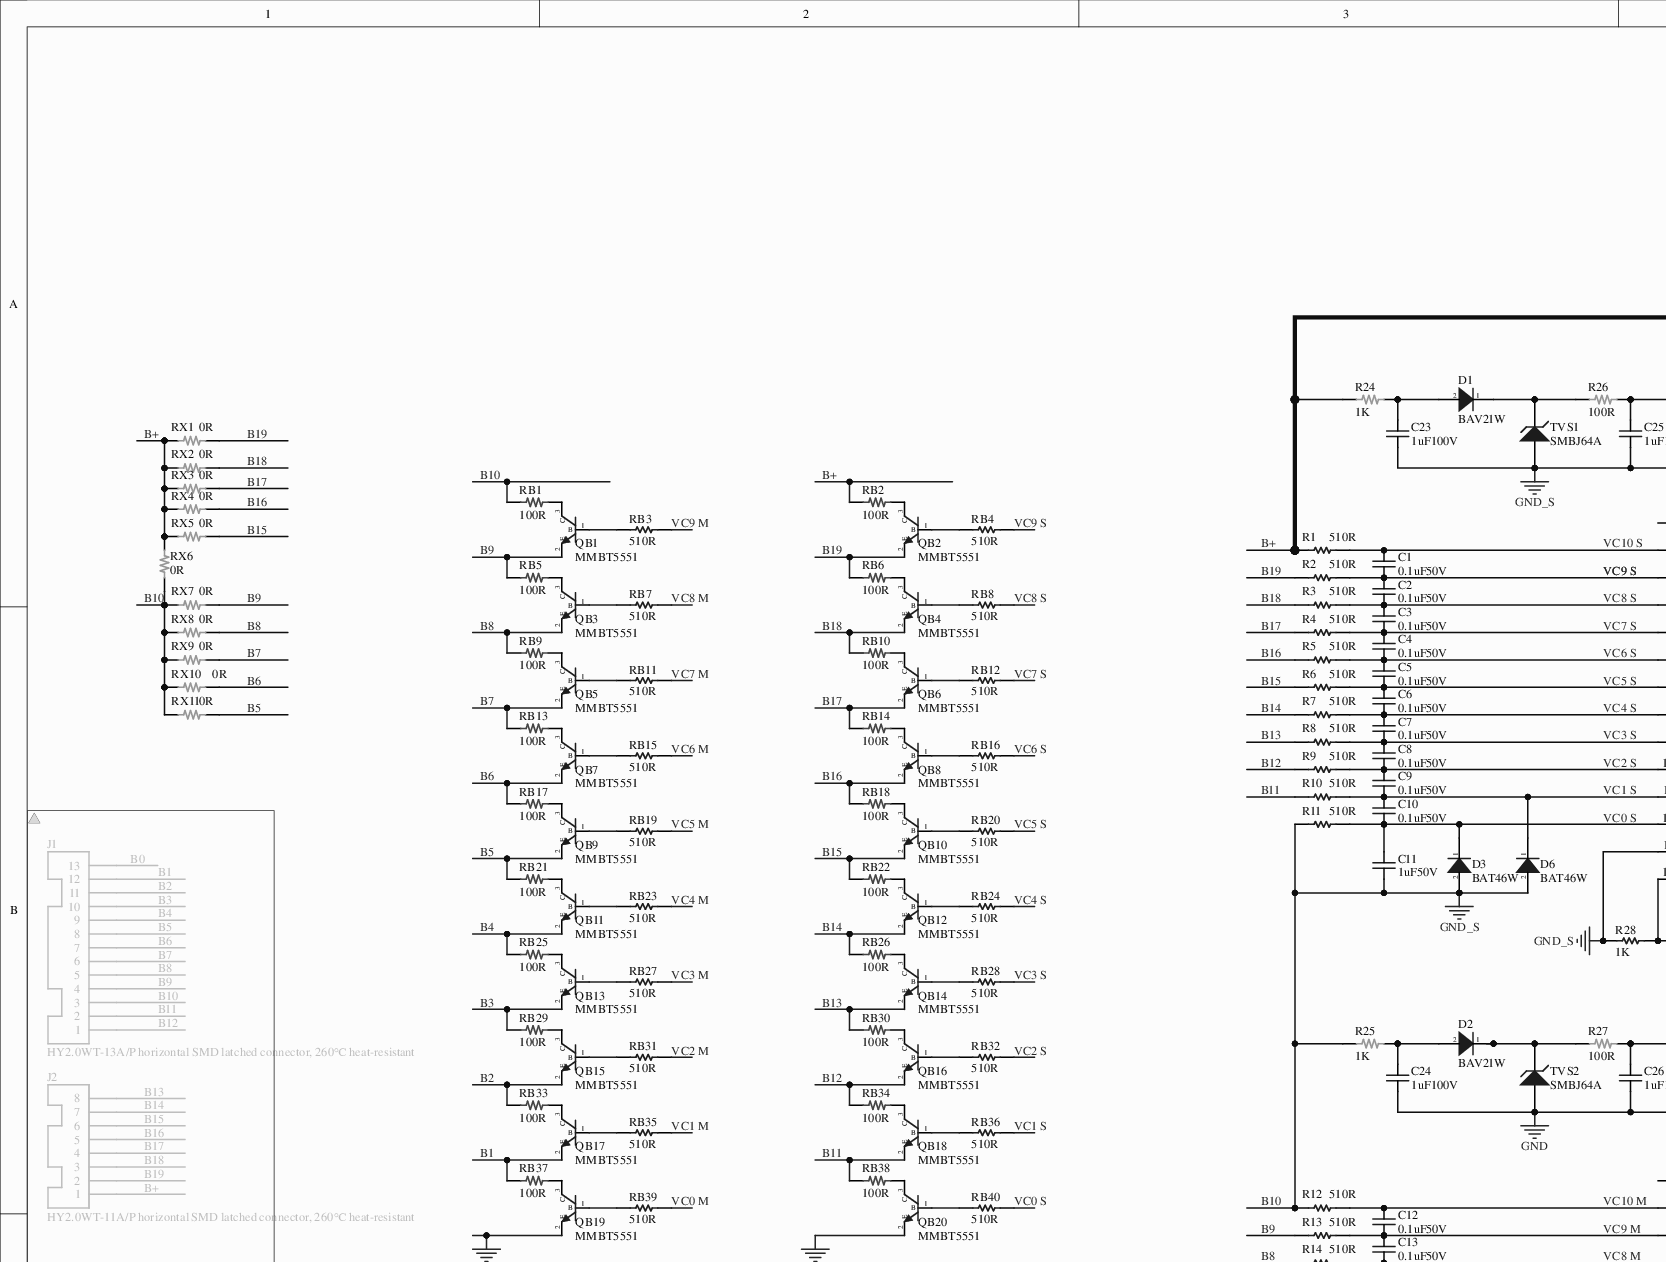
[diagram p0: MISC82749.SchDoc, top left]
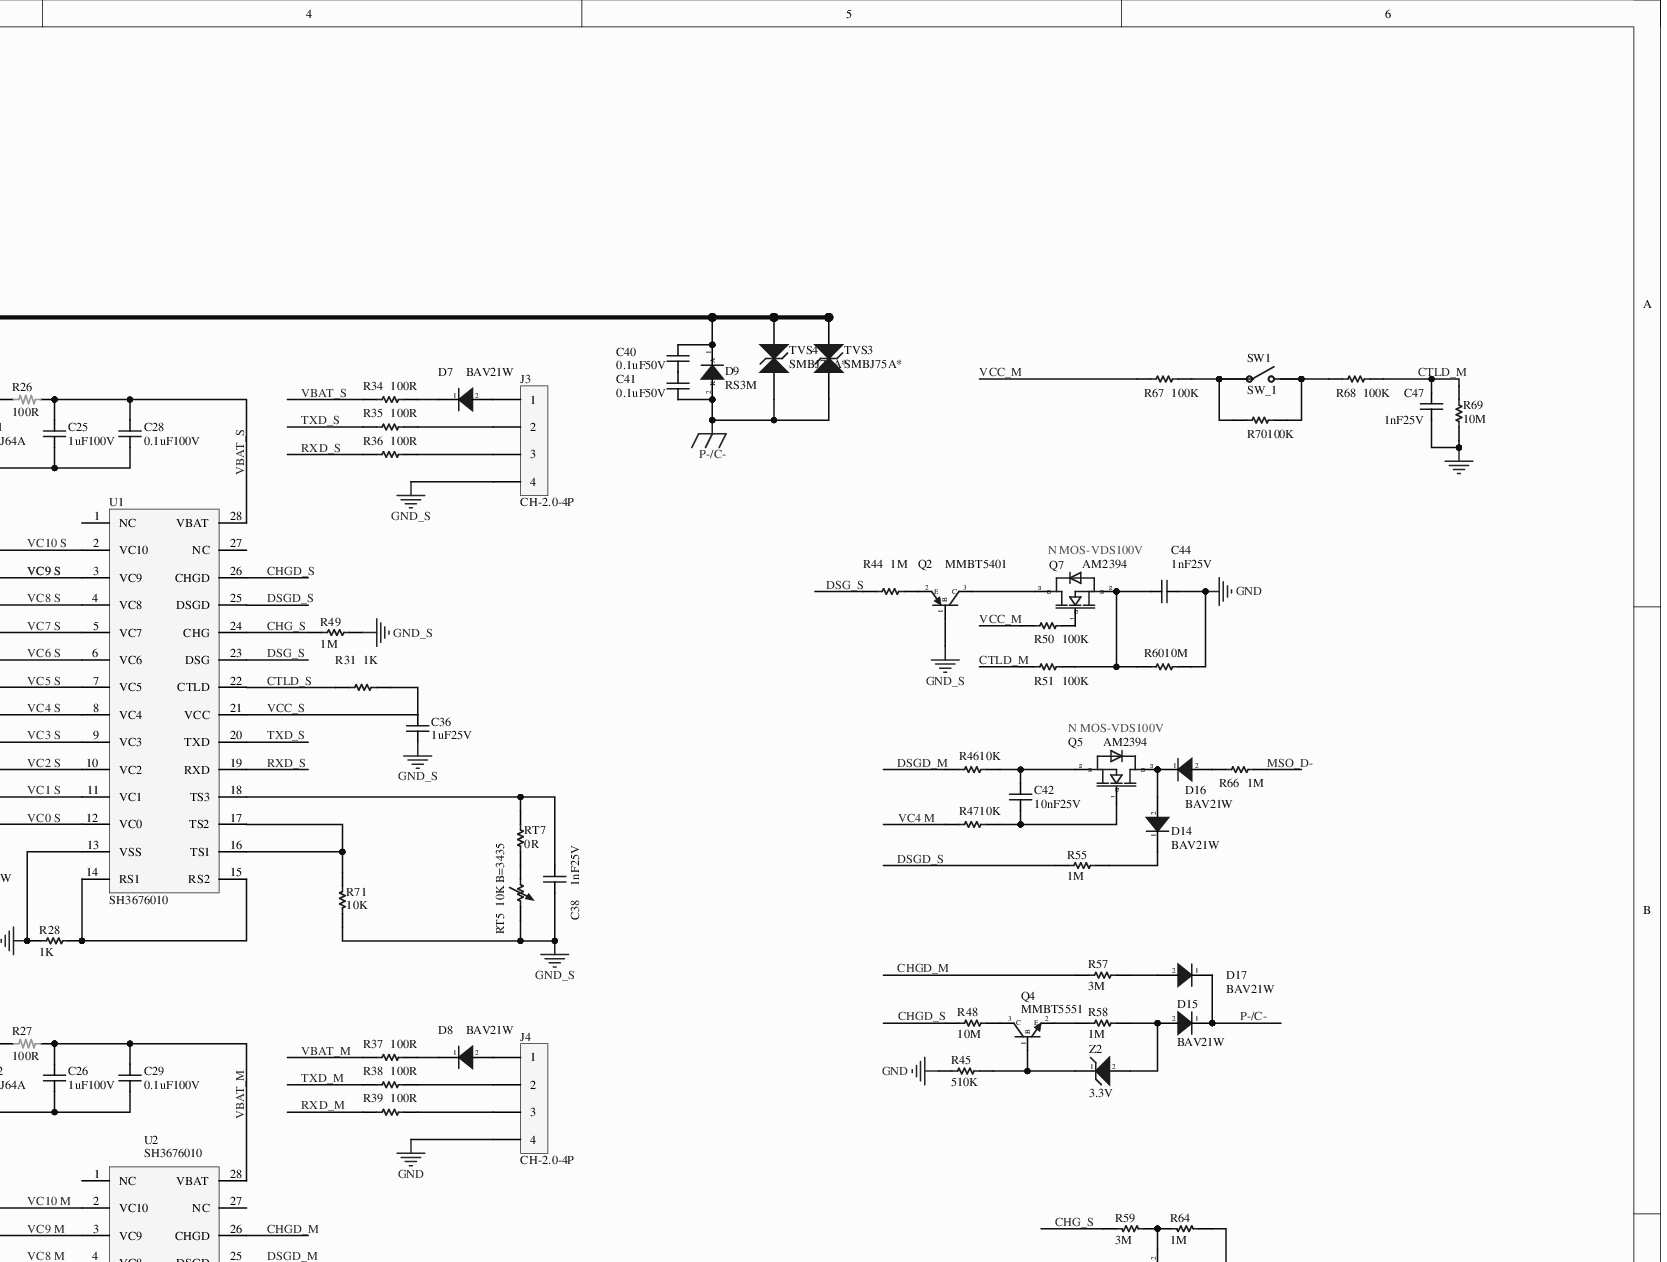
[diagram p1: MISC82749.SchDoc, top right]
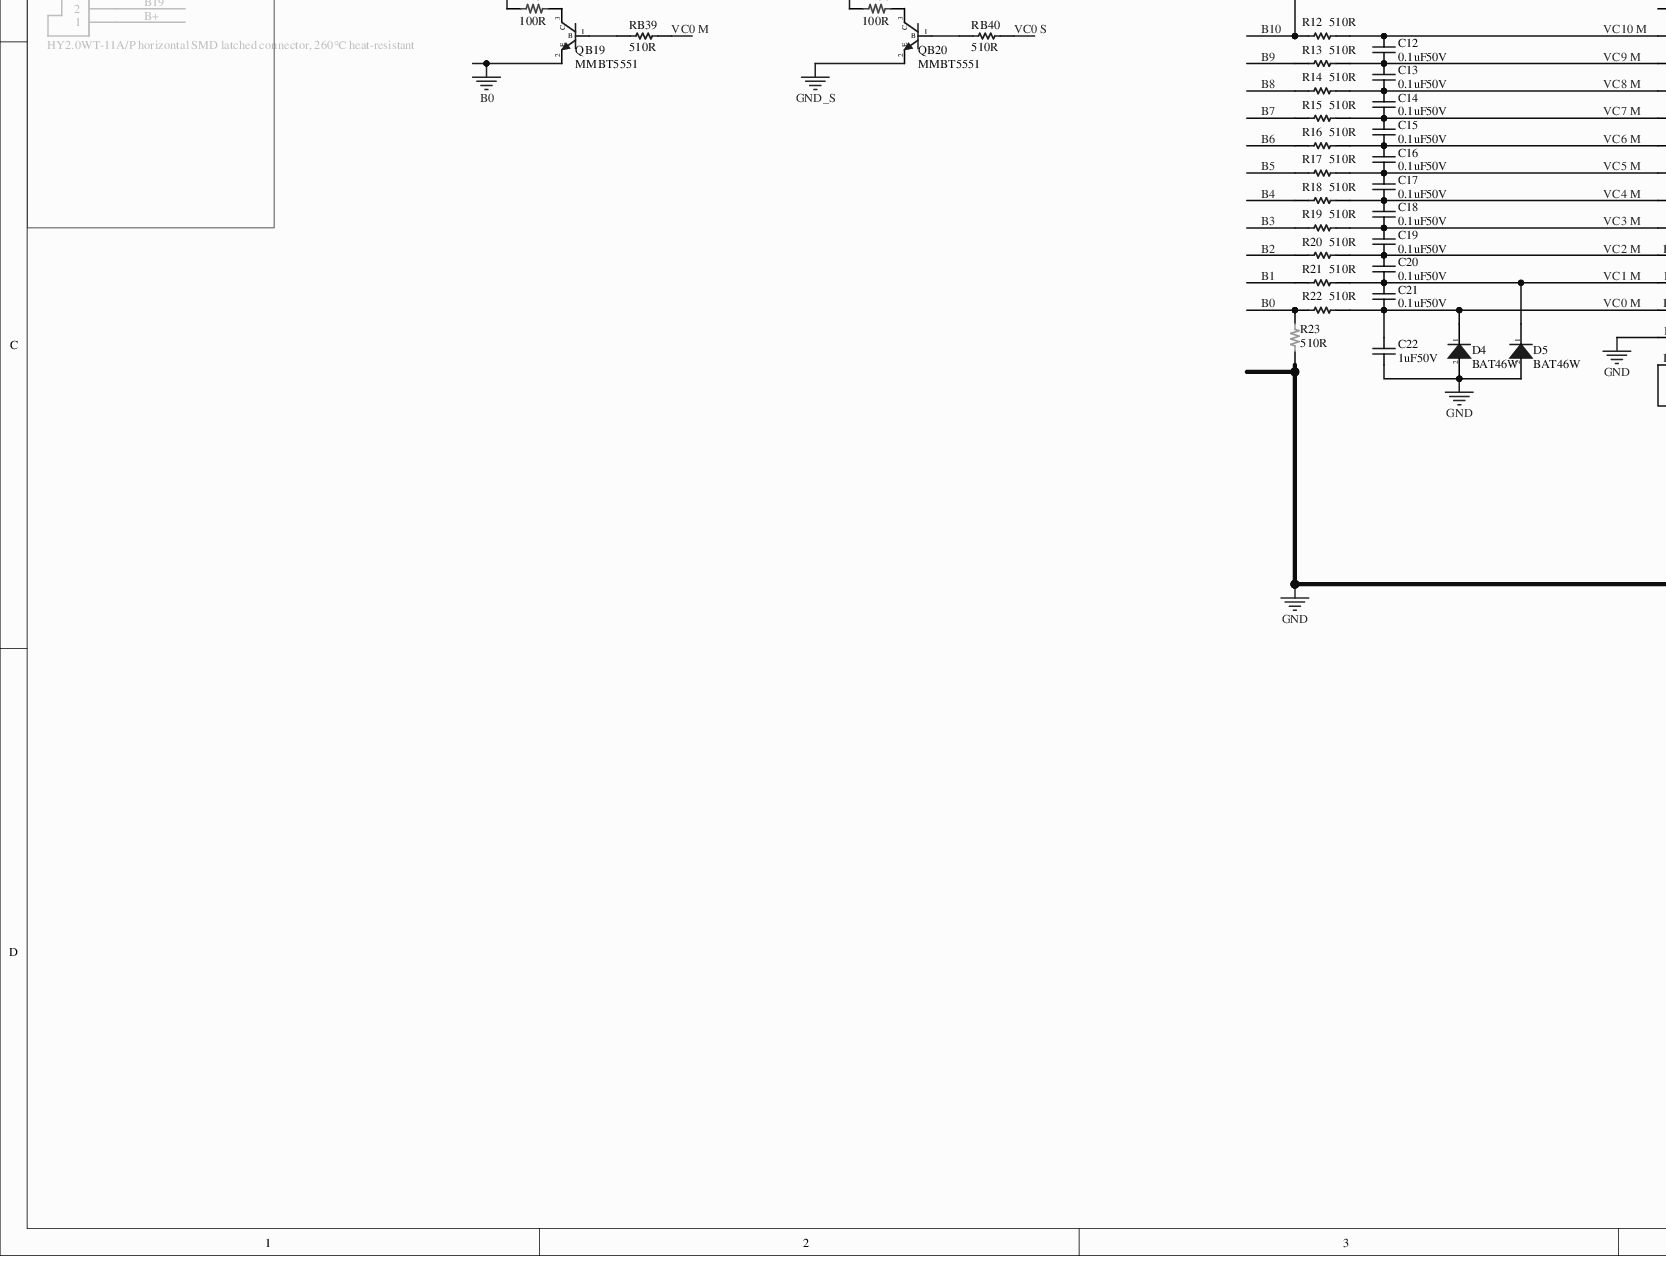
[diagram p2: MISC82749.SchDoc, bottom left]
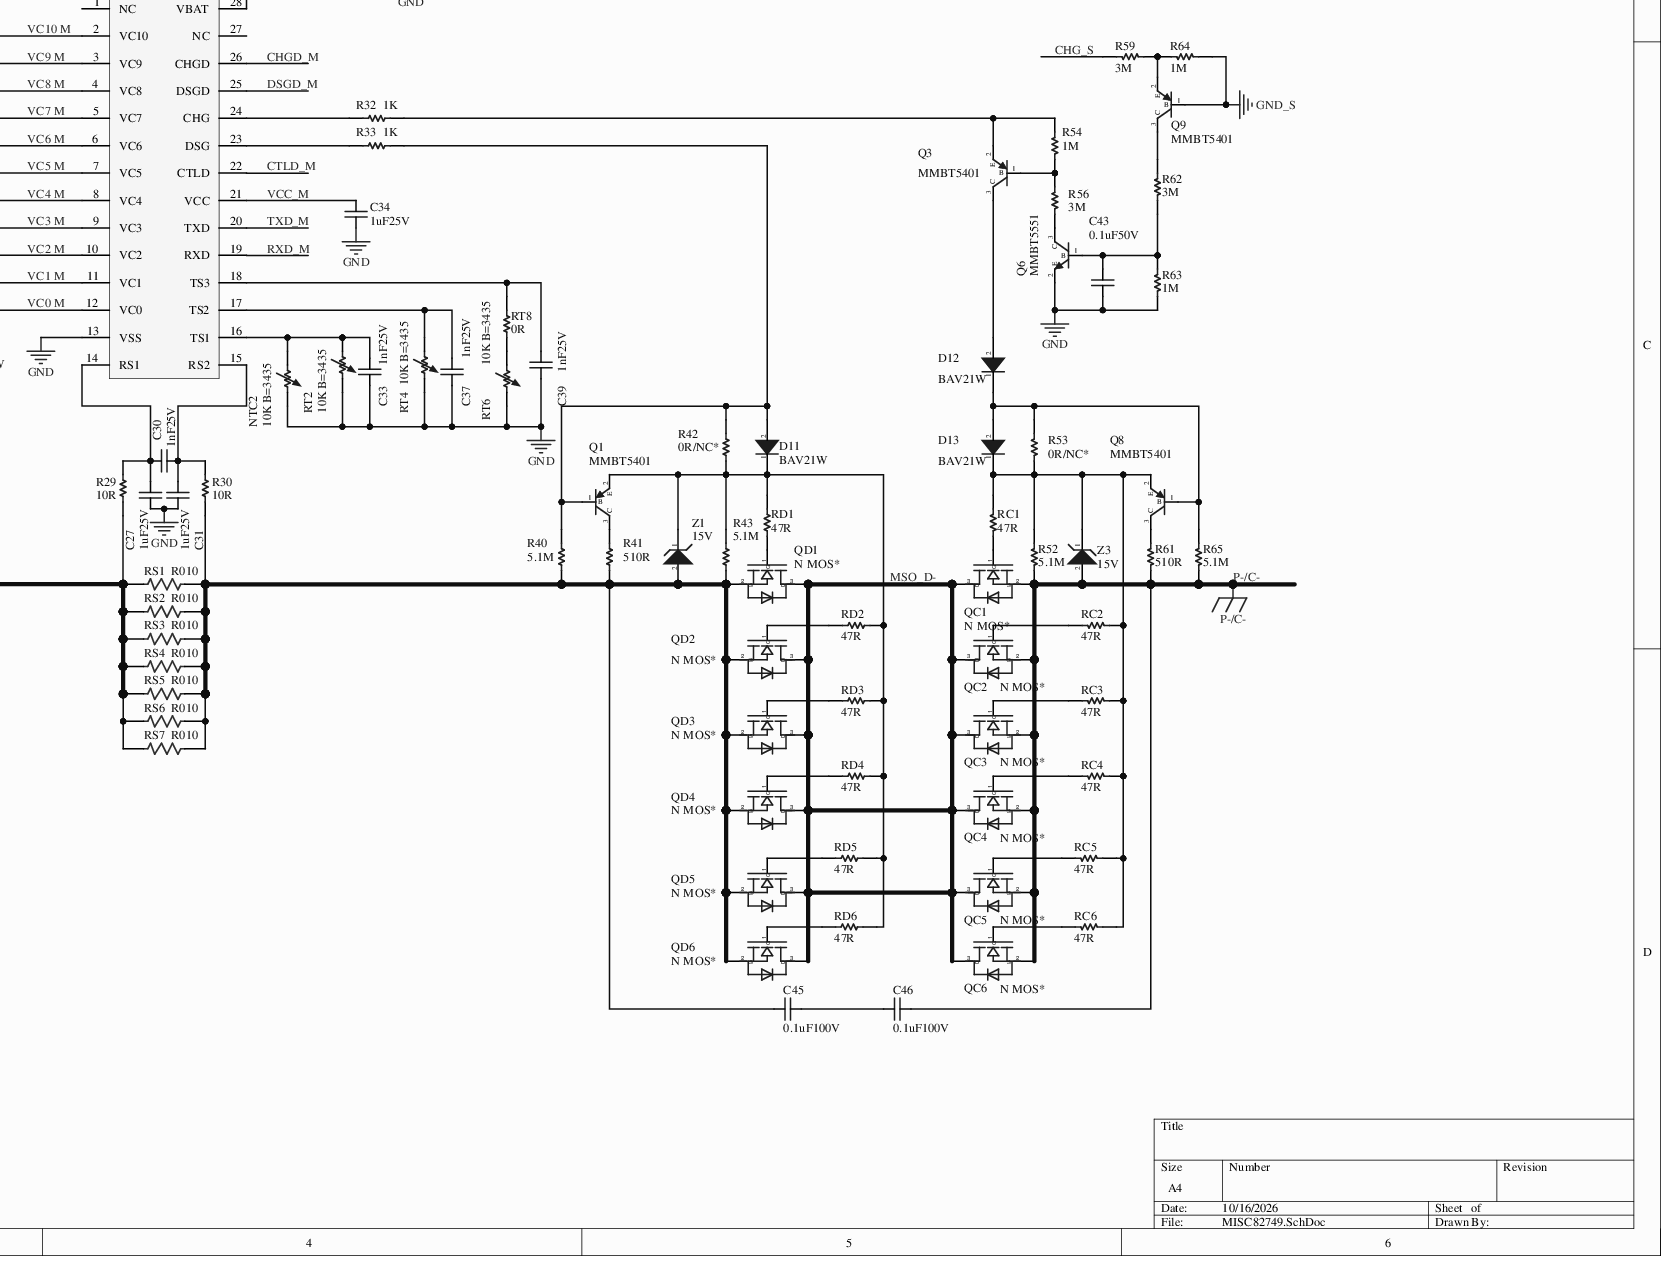
[diagram p3: MISC82749.SchDoc, bottom right]
# Altium project MISC82749.PrjPcb
1 sheet, 264 parts. Net scope: global (net labels, ports and power ports of the same name join across sheets).
Board file: MISC82749.PcbDoc

## Sheet MISC82749.SchDoc
size 599 x 449 mm; SheetNumber: 1; SheetTotal: 1

### Parts
C1  0.1uF50V  [C0603A]
C2  0.1uF50V  [C0603A]
C3  0.1uF50V  [C0603A]
C4  0.1uF50V  [C0603A]
C5  0.1uF50V  [C0603A]
C6  0.1uF50V  [C0603A]
C7  0.1uF50V  [C0603A]
C8  0.1uF50V  [C0603A]
C9  0.1uF50V  [C0603A]
C10  0.1uF50V  [C0603A]
C11  1uF50V  [C0603A]
C12  0.1uF50V  [C0603A]
C13  0.1uF50V  [C0603A]
C14  0.1uF50V  [C0603A]
C15  0.1uF50V  [C0603A]
C16  0.1uF50V  [C0603A]
C17  0.1uF50V  [C0603A]
C18  0.1uF50V  [C0603A]
C19  0.1uF50V  [C0603A]
C20  0.1uF50V  [C0603A]
C21  0.1uF50V  [C0603A]
C22  1uF50V  [C0603A]
C23  1uF100V  [C0805L]
C24  1uF100V  [C0805L]
C25  1uF100V  [C0805L]
C26  1uF100V  [C0805L]
C27  1uF25V  [C0603A]
C28  0.1uF100V  [C0805L]
C29  0.1uF100V  [C0805L]
C30  1nF25V  [C0603A]
C31  1uF25V  [C0603A]
C33  1nF25V  [C0603A]
C34  1uF25V  [C0603A]
C36  1uF25V  [C0603A]
C37  1nF25V  [C0603A]
C38  1nF25V  [C0603A]
C39  1nF25V  [C0603A]
C40  0.1uF50V  [C0603A]
C41  0.1uF50V  [C0603A]
C42  10nF25V  [C0603A]
C43  0.1uF50V  [C0603A]
C44  1nF25V  [C0603A]
C45  0.1uF100V  [C0603A]
C46  0.1uF100V  [C0603A]
C47  1nF25V  [C0603A]
D1  BAV21W  [SOD323A]
D2  BAV21W  [SOD323A]
D3  BAT46W  [SOD123]
D4  BAT46W  [SOD123]
D5  BAT46W  [SOD123]
D6  BAT46W  [SOD123]
D7  BAV21W  [SOD323A]
D8  BAV21W  [SOD323A]
D9  RS3M  [SMB A]
D11  BAV21W  [SOD323A]
D12  BAV21W  [SOD323A]
D13  BAV21W  [SOD323A]
D14  BAV21W  [SOD323A]
D15  BAV21W  [SOD323A]
D16  BAV21W  [SOD323A]
D17  BAV21W  [SOD323A]
J1  HY2.0WT-13A/P horizontal SMD latched connector, 260℃ heat-resistant  [2.0-13PIN直针带扣连接器]  (masked out: inside a compile mask, not in the netlist)
J2  HY2.0WT-11A/P horizontal SMD latched connector, 260℃ heat-resistant  [2.0-8PIN直针带扣连接器]  (masked out: inside a compile mask, not in the netlist)
J3  CH-2.0-4P  [Test2.0-4P]
J4  CH-2.0-4P  [Test2.0-4P]
NTC2  10K B=3435  [RT2.3X1.2-2]
Q1  MMBT5401  [SOT23-3]
Q2  MMBT5401  [SOT23-3]
Q3  MMBT5401  [SOT23-3]
Q4  MMBT5551  [SOT23-3]
Q5  AM2394  [SOT23-3L]
Q6  MMBT5551  [SOT23-3]
Q7  AM2394  [SOT23-3L]
Q8  MMBT5401  [SOT23-3]
Q9  MMBT5401  [SOT23-3]
QB1  MMBT5551  [SOT23-3]
QB2  MMBT5551  [SOT23-3]
QB3  MMBT5551  [SOT23-3]
QB4  MMBT5551  [SOT23-3]
QB5  MMBT5551  [SOT23-3]
QB6  MMBT5551  [SOT23-3]
QB7  MMBT5551  [SOT23-3]
QB8  MMBT5551  [SOT23-3]
QB9  MMBT5551  [SOT23-3]
QB10  MMBT5551  [SOT23-3]
QB11  MMBT5551  [SOT23-3]
QB12  MMBT5551  [SOT23-3]
QB13  MMBT5551  [SOT23-3]
QB14  MMBT5551  [SOT23-3]
QB15  MMBT5551  [SOT23-3]
QB16  MMBT5551  [SOT23-3]
QB17  MMBT5551  [SOT23-3]
QB18  MMBT5551  [SOT23-3]
QB19  MMBT5551  [SOT23-3]
QB20  MMBT5551  [SOT23-3]
QC1  N MOS*  [TOLL_123]
QC2  N MOS*  [TOLL_123]
QC3  N MOS*  [TOLL_123]
QC4  N MOS*  [TOLL_123]
QC5  N MOS*  [TOLL_123]
QC6  N MOS*  [TOLL_123]
QD1  N MOS*  [TOLL_123]
QD2  N MOS*  [TOLL_123]
QD3  N MOS*  [TOLL_123]
QD4  N MOS*  [TOLL_123]
QD5  N MOS*  [TOLL_123]
QD6  N MOS*  [TOLL_123]
R1  510R  [R0603A]
R2  510R  [R0603A]
R3  510R  [R0603A]
R4  510R  [R0603A]
R5  510R  [R0603A]
R6  510R  [R0603A]
R7  510R  [R0603A]
R8  510R  [R0603A]
R9  510R  [R0603A]
R10  510R  [R0603A]
R11  510R  [R0603A]
R12  510R  [R0603A]
R13  510R  [R0603A]
R14  510R  [R0603A]
R15  510R  [R0603A]
R16  510R  [R0603A]
R17  510R  [R0603A]
R18  510R  [R0603A]
R19  510R  [R0603A]
R20  510R  [R0603A]
R21  510R  [R0603A]
R22  510R  [R0603A]
R23  510R  [R0805L]
R24  1K  [R0805L]
R25  1K  [R0805L]
R26  100R  [R0805L]
R27  100R  [R0805L]
R28  1K  [R0603A]
R29  10R  [R0603A]
R30  10R  [R0603A]
R31  1K  [R0603A]
R32  1K  [R0603A]
R33  1K  [R0603A]
R34  100R  [R0603A]
R35  100R  [R0603A]
R36  100R  [R0603A]
R37  100R  [R0603A]
R38  100R  [R0603A]
R39  100R  [R0603A]
R40  5.1M  [R0603A]
R41  510R  [R0603A]
R42  0R/NC*  [R0603A]
R43  5.1M  [R0603A]
R44  1M  [R0603A]
R45  510K  [R0603A]
R46  10K  [R0603A]
R47  10K  [R0603A]
R48  10M  [R0603A]
R49  1M  [R0603A]
R50  100K  [R0603A]
R51  100K  [R0603A]
R52  5.1M  [R0603A]
R53  0R/NC*  [R0603A]
R54  1M  [R0603A]
R55  1M  [R0603A]
R56  3M  [R0603A]
R57  3M  [R0603A]
R58  1M  [R0603A]
R59  3M  [R0603A]
R60  10M  [R0603A]
R61  510R  [R0603A]
R62  3M  [R0603A]
R63  1M  [R0603A]
R64  1M  [R0603A]
R65  5.1M  [R0603A]
R66  1M  [R0603A]
R67  100K  [R0603A]
R68  100K  [R0603A]
R69  10M  [R0603A]
R70  100K  [R0603A]
R71  10K  [R0603A]
RB1  100R  [R1206A]
RB2  100R  [R1206A]
RB3  510R  [R0603A]
RB4  510R  [R0603A]
RB5  100R  [R1206A]
RB6  100R  [R1206A]
RB7  510R  [R0603A]
RB8  510R  [R0603A]
RB9  100R  [R1206A]
RB10  100R  [R1206A]
RB11  510R  [R0603A]
RB12  510R  [R0603A]
RB13  100R  [R1206A]
RB14  100R  [R1206A]
RB15  510R  [R0603A]
RB16  510R  [R0603A]
RB17  100R  [R1206A]
RB18  100R  [R1206A]
RB19  510R  [R0603A]
RB20  510R  [R0603A]
RB21  100R  [R1206A]
RB22  100R  [R1206A]
RB23  510R  [R0603A]
RB24  510R  [R0603A]
RB25  100R  [R1206A]
RB26  100R  [R1206A]
RB27  510R  [R0603A]
RB28  510R  [R0603A]
RB29  100R  [R1206A]
RB30  100R  [R1206A]
RB31  510R  [R0603A]
RB32  510R  [R0603A]
RB33  100R  [R1206A]
RB34  100R  [R1206A]
RB35  510R  [R0603A]
RB36  510R  [R0603A]
RB37  100R  [R1206A]
RB38  100R  [R1206A]
RB39  510R  [R0603A]
RB40  510R  [R0603A]
RC1  47R  [R0603A]
RC2  47R  [R0603A]
RC3  47R  [R0603A]
RC4  47R  [R0603A]
RC5  47R  [R0603A]
RC6  47R  [R0603A]
RD1  47R  [R0603A]
RD2  47R  [R0603A]
RD3  47R  [R0603A]
RD4  47R  [R0603A]
RD5  47R  [R0603A]
RD6  47R  [R0603A]
RS1  R010  [R2512L]
RS2  R010  [R2512L]
RS3  R010  [R2512L]
RS4  R010  [R2512L]
RS5  R010  [R2512L]
RS6  R010  [R2512L]
RS7  R010  [R2512L]
RT2  10K B=3435  [R0603A]
RT4  10K B=3435  [R0603A]
RT5  10K B=3435  [R0603A]
RT6  10K B=3435  [R0603A]
RT7  0R  [R0603A]
RT8  0R  [R0603A]
RX1  0R  [R0805L]
RX2  0R  [R0805L]
RX3  0R  [R0805L]
RX4  0R  [R0805L]
RX5  0R  [R0805L]
RX6  0R  [R0805L]
RX7  0R  [R0805L]
RX8  0R  [R0805L]
RX9  0R  [R0805L]
RX10  0R  [R0805L]
RX11  0R  [R0805L]
SW1  SW_1  [RT2.3X1.2-2]
TVS1  SMBJ64A  [SMB A]
TVS2  SMBJ64A  [SMB A]
TVS3  SMBJ75A*  [SMC_MDO-214AB)]
TVS4  SMBJ75A*  [SMC_MDO-214AB)]
U1  SH3676010  [TSSOP-28L(PIN间距0.65mm)]
U2  SH3676010  [TSSOP-28L(PIN间距0.65mm)]
Z1  15V  [SOD323A]
Z2  3.3V  [SOD323A]
Z3  15V  [SOD323A]

### Nets
B0: QB19.2(E) R22.1 R23.2
B10: C11.1 C23.1 C25.1 C28.1 C36.1 C38.2 D3.2(K) D6.2(K) J3.4 Q2.1(B) Q9.1(B) QB20.2(E) R11.1 R12.1 R25.2 R28.1 R49.2 R64.2 R71.1 RB1.1 RT5.2 RX6.1 RX7.1 RX8.1 RX9.1 RX10.1 RX11.1 TVS1.2(K) U1.13(VSS)  [also labelled GND_S]
GND: C22.1 C24.1 C26.1 C27.2 C29.1 C31.1 C33.2 C34.1 C37.2 C39.2 C43.1 C44.2 C47.1 D4.2(K) D5.2(K) J4.4 NTC2.2 Q6.2(E) R23.1 R29.1 R45.1 R60.1 R63.2 R69.2 RS1.1 RS2.1 RS3.1 RS4.1 RS5.1 RS6.1 RS7.1 RT2.2 RT4.2 RT6.2 TVS2.2(K) U2.13(VSS)
P-/C-: C41.1 C46.1 D9.2(K) D15.1(A) D17.1(A) QC1.2(S) QC2.2(S) QC3.2(S) QC4.2(S) QC5.2(S) QC6.2(S) R52.2 R61.2 R65.2 TVS3.1(A) TVS4.1(A) Z3.2(K)
B1: QB17.2(E) R21.1 RB37.1
B2: QB15.2(E) R20.1 RB33.1
B3: QB13.2(E) R19.1 RB29.1
B4: QB11.2(E) R18.1 RB25.1
B5: QB9.2(E) R17.1 RB21.1 RX11.2
B6: QB7.2(E) R16.1 RB17.1 RX10.2
B7: QB5.2(E) R15.1 RB13.1 RX9.2
B8: QB3.2(E) R14.1 RB9.1 RX8.2
B9: QB1.2(E) R13.1 RB5.1 RX7.2
B11: QB18.2(E) R10.1 RB38.1
B12: QB16.2(E) R9.1 RB34.1
B13: QB14.2(E) R8.1 RB30.1
B14: QB12.2(E) R7.1 RB26.1
B15: QB10.2(E) R6.1 RB22.1 RX5.2
B16: QB8.2(E) R5.1 RB18.1 RX4.2
B17: QB6.2(E) R4.1 RB14.1 RX3.2
B18: QB4.2(E) R3.1 RB10.1 RX2.2
B19: QB2.2(E) R2.1 RB6.1 RX1.2
B+: C40.2 D9.1(A) R1.1 R24.2 RB2.1 RX1.1 RX2.1 RX3.1 RX4.1 RX5.1 RX6.2 TVS3.2(K) TVS4.2(K)
CHG_S: R49.1 R59.2 U1.24(CHG)
CHGD_M: R57.2 U2.26(CHGD)
CHGD_S: R48.2 U1.26(CHGD)
CTLD_M: C47.2 R51.2 R68.1 R69.1 U2.22(CTLD)
CTLD_S: R31.2 U1.22(CTLD)
DSG_S: R44.2 U1.23(DSG)
DSGD_M: R46.2 U2.25(DSGD)
DSGD_S: R55.2 U1.25(DSGD)
MSO_D-: QC1.3(D) QC2.3(D) QC3.3(D) QC4.3(D) QC5.3(D) QC6.3(D) QD1.3(D) QD2.3(D) QD3.3(D) QD4.3(D) QD5.3(D) QD6.3(D) R66.1
RXD_M: R39.1 U2.19(RXD)
RXD_S: R36.1 U1.19(RXD)
TXD_M: R38.1 U2.20(TXD)
TXD_S: R35.1 U1.20(TXD)
VBAT_M: C26.2 C29.2 R27.1 R37.1 U2.28(VBAT)
VBAT_S: C25.2 C28.2 R26.1 R34.1 U1.28(VBAT)
VC0 M: C21.1 C22.2 D4.1(A) R22.2 RB39.2 U2.12(VC0)
VC0 S: C10.1 C11.2 D3.1(A) R11.2 RB40.2 U1.12(VC0)
VC1 M: C20.1 C21.2 D5.1(A) R21.2 RB35.2 U2.11(VC1)
VC1 S: C9.1 C10.2 D6.1(A) R10.2 RB36.2 U1.11(VC1)
VC2 M: C19.1 C20.2 R20.2 RB31.2 U2.10(VC2)
VC2 S: C8.1 C9.2 R9.2 RB32.2 U1.10(VC2)
VC3 M: C18.1 C19.2 R19.2 RB27.2 U2.9(VC3)
VC3 S: C7.1 C8.2 R8.2 RB28.2 U1.9(VC3)
VC4 M: C17.1 C18.2 R18.2 R47.2 RB23.2 U2.8(VC4)
VC4 S: C6.1 C7.2 R7.2 RB24.2 U1.8(VC4)
VC5 M: C16.1 C17.2 R17.2 RB19.2 U2.7(VC5)
VC5 S: C5.1 C6.2 R6.2 RB20.2 U1.7(VC5)
VC6 M: C15.1 C16.2 R16.2 RB15.2 U2.6(VC6)
VC6 S: C4.1 C5.2 R5.2 RB16.2 U1.6(VC6)
VC7 M: C14.1 C15.2 R15.2 RB11.2 U2.5(VC7)
VC7 S: C3.1 C4.2 R4.2 RB12.2 U1.5(VC7)
VC8 M: C13.1 C14.2 R14.2 RB7.2 U2.4(VC8)
VC8 S: C2.1 C3.2 R3.2 RB8.2 U1.4(VC8)
VC9 M: C12.1 C13.2 R13.2 RB3.2 U2.3(VC9)
VC9 S: C1.1 C2.2 R2.2 RB4.2 U1.3(VC9)
VC10 M: C12.2 R12.2 U2.2(VC10)
VC10 S: C1.2 R1.2 U1.2(VC10)
VCC_M: C34.2 R50.2 R67.2 U2.21(VCC)
VCC_S: C36.2 R31.1 U1.21(VCC)
NetC23_2: C23.2 D1.2(K) R24.1
NetC24_2: C24.2 D2.2(K) R25.1
NetC27_1: C27.1 C30.2 R29.2 U2.14(RS1)
NetC30_1: C30.1 C31.2 R30.1 U2.15(RS2)
NetC33_1: C33.1 NTC2.1 RT2.1 U2.16(TS1)
NetC37_1: C37.1 RT4.1 U2.17(TS2)
NetC38_1: C38.1 RT7.2 U1.18(TS3)
NetC39_1: C39.1 RT8.2 U2.18(TS3)
NetC40_1: C40.1 C41.2
NetC42_1: C42.1 Q5.1(G) R47.1
NetC42_2: C42.2 Q5.2(S) R46.1
NetC43_2: C43.2 Q6.1(B) R62.1 R63.1
NetC44_1: C44.1 Q7.2(S) R51.1 R60.2
NetC45_1: C45.1 C46.2
NetC45_2: C45.2 QD1.2(S) QD2.2(S) QD3.2(S) QD4.2(S) QD5.2(S) QD6.2(S) R30.2 R40.2 R41.2 R43.2 RS1.2 RS2.2 RS3.2 RS4.2 RS5.2 RS6.2 RS7.2 Z1.2(K)
NetD1_1: D1.1(A) R26.2 TVS1.1(A)
NetD2_1: D2.1(A) R27.2 TVS2.1(A)
NetD7_1: D7.1(A) R34.2
NetD7_2: D7.2(K) J3.1
NetD8_1: D8.1(A) R37.2
NetD8_2: D8.2(K) J4.1
NetD11_1: D11.1(A) Q1.2(E) R42.2 R43.1 RD1.1 RD2.1 RD3.1 RD4.2 RD5.2 RD6.2 Z1.1(A)
NetD11_2: D11.2(K) Q1.1(B) R33.2 R40.1 R42.1
NetD12_1: D12.1(A) D13.2(K) Q8.1(B) R53.1 R65.1
NetD12_2: D12.2(K) Q3.3(C)
NetD13_1: D13.1(A) Q8.2(E) R52.1 R53.2 RC1.1 RC2.2 RC3.2 RC4.1 RC5.1 RC6.1 Z3.1(A)
NetD14_1: D14.1(A) R55.1
NetD14_2: D14.2(K) D16.1(A) Q5.3(D)
NetD15_2: D15.2(K) R58.1 Z2.2(K)
NetD16_2: D16.2(K) R66.2
NetD17_2: D17.2(K) R57.1
NetJ3_2: J3.2 R35.2
NetJ3_3: J3.3 R36.2
NetJ4_2: J4.2 R38.2
NetJ4_3: J4.3 R39.2
NetQ1_3: Q1.3(C) R41.1
NetQ2_2: Q2.2(E) R44.1
NetQ2_3: Q2.3(C) Q7.3(D)
NetQ3_1: Q3.1(B) R54.1 R56.1
NetQ3_2: Q3.2(E) R32.2 R54.2
NetQ4_1: Q4.1(B) R45.2 Z2.1(A)
NetQ4_2: Q4.2(E) R58.2
NetQ4_3: Q4.3(C) R48.1
NetQ6_3: Q6.3(C) R56.2
NetQ7_1: Q7.1(G) R50.1
NetQ8_3: Q8.3(C) R61.1
NetQ9_2: Q9.2(E) R59.1 R64.1
NetQ9_3: Q9.3(C) R62.2
NetQB1_1: QB1.1(B) RB3.1
NetQB1_3: QB1.3(C) RB1.2
NetQB2_1: QB2.1(B) RB4.1
NetQB2_3: QB2.3(C) RB2.2
NetQB3_1: QB3.1(B) RB7.1
NetQB3_3: QB3.3(C) RB5.2
NetQB4_1: QB4.1(B) RB8.1
NetQB4_3: QB4.3(C) RB6.2
NetQB5_1: QB5.1(B) RB11.1
NetQB5_3: QB5.3(C) RB9.2
NetQB6_1: QB6.1(B) RB12.1
NetQB6_3: QB6.3(C) RB10.2
NetQB7_1: QB7.1(B) RB15.1
NetQB7_3: QB7.3(C) RB13.2
NetQB8_1: QB8.1(B) RB16.1
NetQB8_3: QB8.3(C) RB14.2
NetQB9_1: QB9.1(B) RB19.1
NetQB9_3: QB9.3(C) RB17.2
NetQB10_1: QB10.1(B) RB20.1
NetQB10_3: QB10.3(C) RB18.2
NetQB11_1: QB11.1(B) RB23.1
NetQB11_3: QB11.3(C) RB21.2
NetQB12_1: QB12.1(B) RB24.1
NetQB12_3: QB12.3(C) RB22.2
NetQB13_1: QB13.1(B) RB27.1
NetQB13_3: QB13.3(C) RB25.2
NetQB14_1: QB14.1(B) RB28.1
NetQB14_3: QB14.3(C) RB26.2
NetQB15_1: QB15.1(B) RB31.1
NetQB15_3: QB15.3(C) RB29.2
NetQB16_1: QB16.1(B) RB32.1
NetQB16_3: QB16.3(C) RB30.2
NetQB17_1: QB17.1(B) RB35.1
NetQB17_3: QB17.3(C) RB33.2
NetQB18_1: QB18.1(B) RB36.1
NetQB18_3: QB18.3(C) RB34.2
NetQB19_1: QB19.1(B) RB39.1
NetQB19_3: QB19.3(C) RB37.2
NetQB20_1: QB20.1(B) RB40.1
NetQB20_3: QB20.3(C) RB38.2
NetQC1_1: QC1.1(G) RC1.2
NetQC2_1: QC2.1(G) RC2.1
NetQC3_1: QC3.1(G) RC3.1
NetQC4_1: QC4.1(G) RC4.2
NetQC5_1: QC5.1(G) RC5.2
NetQC6_1: QC6.1(G) RC6.2
NetQD1_1: QD1.1(G) RD1.2
NetQD2_1: QD2.1(G) RD2.2
NetQD3_1: QD3.1(G) RD3.2
NetQD4_1: QD4.1(G) RD4.1
NetQD5_1: QD5.1(G) RD5.1
NetQD6_1: QD6.1(G) RD6.1
NetR28_2: R28.2 U1.14(RS1) U1.15(RS2)
NetR32_1: R32.1 U2.24(CHG)
NetR33_1: R33.1 U2.23(DSG)
NetR67_1: R67.1 R70.2 SW1.1(COMMON)
NetR68_2: R68.2 R70.1 SW1.2(NO)
NetR71_2: R71.2 U1.16(TS1) U1.17(TS2)
NetRT5_1: RT5.1 RT7.1
NetRT6_1: RT6.1 RT8.1

Not connected (* = marked no-connect by the designer): U1 1(NC)* 27(NC)*; U2 1(NC)* 27(NC)*

### Notes on the sheet
- N MOS-VDS100V

### Library data of the parts
C1-C31 C33 C34 C36-C47 = CAP: SMD capacitor
D1 D2 D7 D8 D11-D17 = BAV21_SOD323: SMD diode
D3-D6 = BAT46W_SOD123: SMD diode
D9 = RS3M: SMD diode
J1 = HY2.0WT-13A/P 卧贴带扣耐温260℃: horizontal SMD latched connector, 260℃ heat-resistant
J2 = HY2.0WT-8A/P 卧贴带扣耐温260℃: horizontal SMD latched connector, 260℃ heat-resistant
J3 J4 = Test2.0-4P: test socket
NTC2 RT2 RT4-RT6 = NTC: SMD thermistor
Q1-Q3 Q8 Q9 = MMBT5401: SMD transistor
Q4 Q6 QB1-QB20 = MMBT5551: SMD transistor
Q5 Q7 = AM2394_VGS100V: SMD N MOS_VGS100V
QC1-QC6 QD1-QD6 = N MOS*: SMD MOSFET
R1-R22 R28-R71 RB3 RB4 RB7 RB8 RB11 RB12 RB15 RB16 RB19 RB20 RB23 RB24 RB27 RB28 RB31 RB32 RB35 RB36 RB39 RB40 RC1-RC6 RD1-RD6 RT7 RT8 = RES: SMD resistor
R23-R27 RX1-RX11 = RES_0805: SMD resistor
RB1 RB2 RB5 RB6 RB9 RB10 RB13 RB14 RB17 RB18 RB21 RB22 RB25 RB26 RB29 RB30 RB33 RB34 RB37 RB38 = RES3: alloy SMD resistor
RS1-RS7 = RES2_2512: SMD alloy resistor
SW1 = SW_1: soft-touch switch
TVS1 TVS2 = SMBJ64A: SMD diode (ESD and surge protection)
TVS3 TVS4 = TVS C: SMD diode (ESD and surge protection)
Z1 Z3 = 15V SOD323: SMD zener diode
Z2 = 3.3_SOD323: SMD zener diode